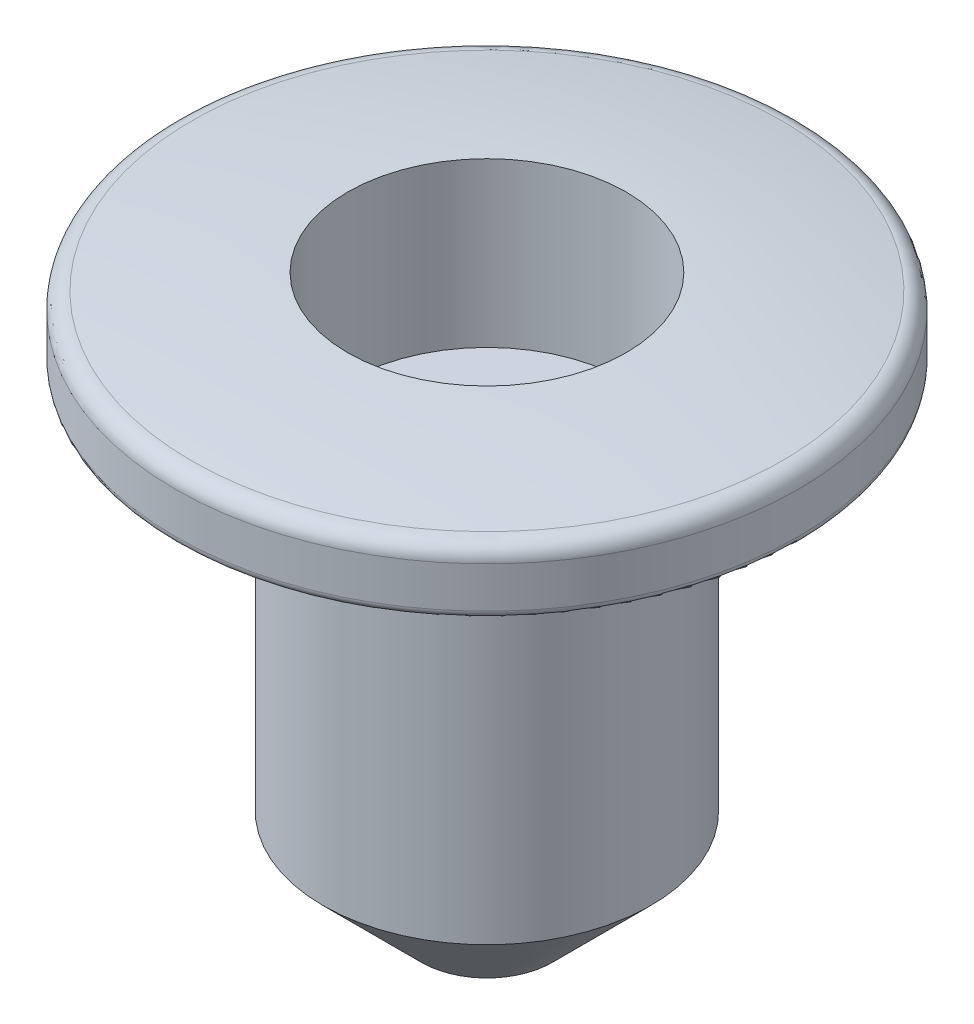
from build123d import *

# Parameters (mm, degrees)
SKETCH3_R          = 2.75
CUT_EXTRUDE1_DEPTH = 10
SKETCH4_R          = 4
CUT_EXTRUDE2_DEPTH = 10


with BuildPart() as part:
    # Sketch1 → Revolve1 (revolve)
    with BuildSketch(Plane.XY, mode=Mode.PRIVATE) as revolve1_sk:
        with BuildLine():
            Line((0, -20), (0, -18.5))
            Line((0, -18.5), (-2.878679656, -18.5))
            Line((-2.878679656, -18.5), (-8.5, -12.878679656))
            Line((-8.5, -12.878679656), (-8.5, 3.5))
            Line((-8.5, 3.5), (-5.5, 3.5))
            Line((-5.5, 3.5), (-5.5, 5))
            Line((-5.5, 5), (-8.5, 5))
            Line((-8.5, 5), (-8.5, 14.977248766))
            ThreePointArc((-8.5, 14.977248766), (-13.264398706, 14.628596634), (-18, 14))
            ThreePointArc((-18, 14), (-18.707106781, 13.707106781), (-19, 13))
            Line((-19, 13), (-19, 10.5))
            ThreePointArc((-19, 10.5), (-18.853553391, 10.146446609), (-18.5, 10))
            Line((-18.5, 10), (-14, 10))
            ThreePointArc((-14, 10), (-11.171572875, 8.828427125), (-10, 6))
            Line((-10, 6), (-10, -13.5))
            Line((-10, -13.5), (-3.5, -20))
            Line((-3.5, -20), (0, -20))
        make_face()
    revolve(revolve1_sk.sketch.rotate(Axis((0, 14, 0), (0, -1, 0)), 270), axis=Axis((0, 14, 0), (0, -1, 0)))

    # Sketch3 → Cut-Extrude1 (cut)
    with BuildSketch(Plane.XZ.offset(20)):
        with Locations(Location((0, 0, 0), (0, 0, 270))):
            Circle(SKETCH3_R)
    extrude(amount=-CUT_EXTRUDE1_DEPTH, mode=Mode.SUBTRACT)

    # Sketch4 → Cut-Extrude2 (cut)
    with BuildSketch(Plane.XZ.offset(20)):
        with Locations(Location((0, 0, 0), (0, 0, 90))):
            Circle(SKETCH4_R)
    extrude(amount=-CUT_EXTRUDE2_DEPTH, mode=Mode.SUBTRACT)


solid = part.part
